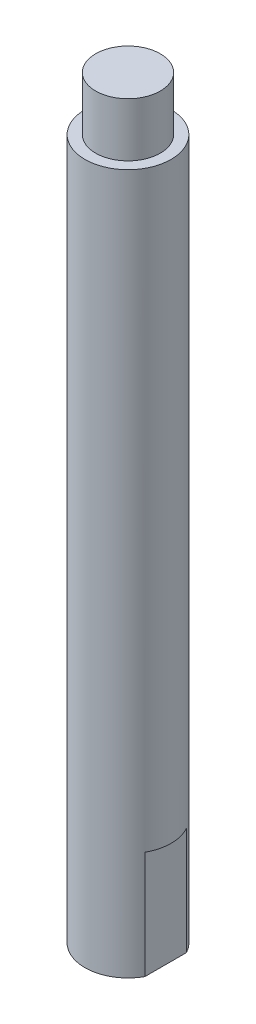
from build123d import *

# Parameters (mm, degrees)
SKETCH1_R           = 8
BOSS_EXTRUDE1_DEPTH = 130
SKETCH4_R           = 6
BOSS_EXTRUDE2_DEPTH = 10
SKETCH5_W           = 13.236787349
SKETCH5_H           = 35.235955056
SKETCH5_W_2         = 13.423220974
SKETCH5_H_2         = 24.946317104
CUT_EXTRUDE1_DEPTH  = 5


with BuildPart() as part:
    # Sketch1 → Boss-Extrude1 (new body)
    with BuildSketch(Plane(origin=(0, 0, 0), x_dir=(1, 0, 0), z_dir=(0, 1, 0))):
        with Locations(Location((0, 0, 0), (0, 0, 270))):
            Circle(SKETCH1_R)
    extrude(amount=BOSS_EXTRUDE1_DEPTH)

    # Sketch4 → Boss-Extrude2 (add)
    with BuildSketch(Plane(origin=(0, 130, 0), x_dir=(1, 0, 0), z_dir=(0, 1, 0))):
        with Locations(Location((0, 0, 0), (0, 0, 270))):
            Circle(SKETCH4_R)
    extrude(amount=BOSS_EXTRUDE2_DEPTH)

    # Sketch5 → Cut-Extrude1 (cut, symmetric)
    with BuildSketch(Plane.XY):
        with Locations((-13.618393675, 2.382022472)):
            Rectangle(SKETCH5_W, SKETCH5_H)
        with Locations((13.711610487, 7.526841448)):
            Rectangle(SKETCH5_W_2, SKETCH5_H_2)
    extrude(amount=CUT_EXTRUDE1_DEPTH, both=True, mode=Mode.SUBTRACT)


solid = part.part
